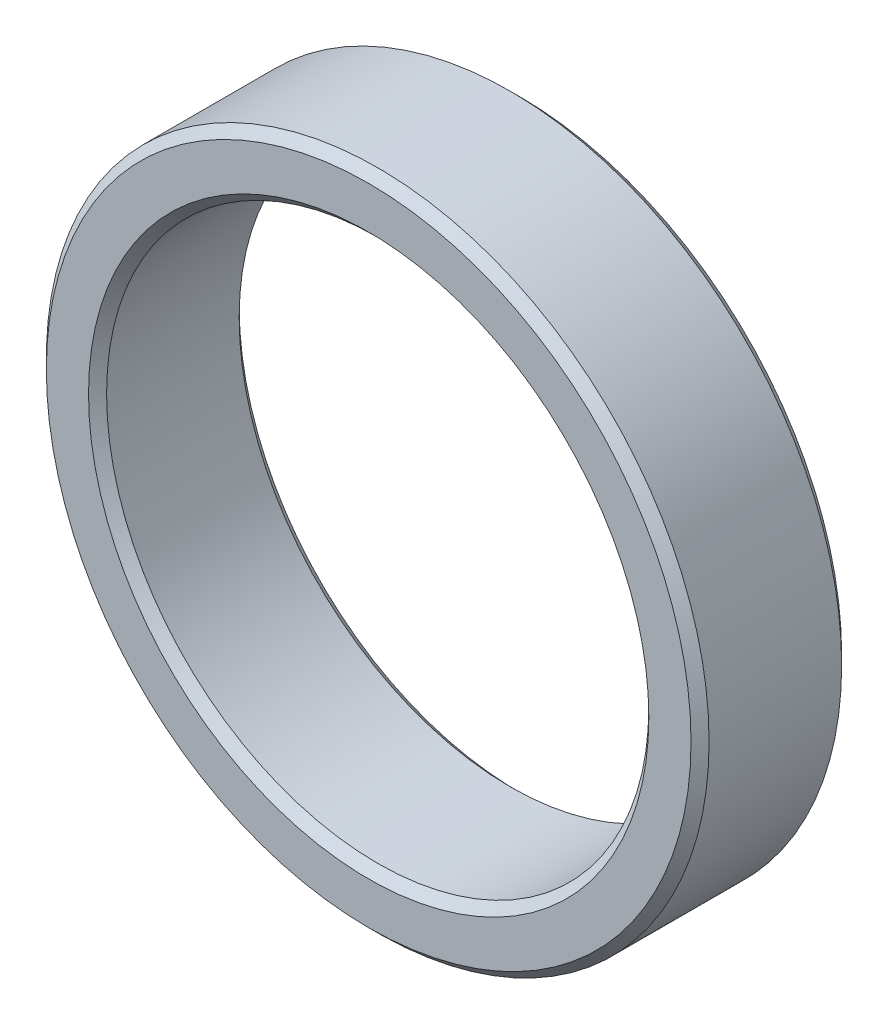
from build123d import *

# Parameters (mm, degrees)
SKETCH_2_R          = 11
EXTRUDE_1_DEPTH     = 5
SKETCH_3_R          = 9
CUT_EXTRUDE_1_DEPTH = 5
CHAMFER_2_SIZE      = 0.3


with BuildPart() as part:
    # 草图2 → 凸台-拉伸1 (new body)
    with BuildSketch(Plane.XY):
        Circle(SKETCH_2_R)
    extrude(amount=EXTRUDE_1_DEPTH)

    # 草图3 → 切除-拉伸1 (cut)
    with BuildSketch(Plane.XY.offset(5)):
        Circle(SKETCH_3_R)
    extrude(amount=-CUT_EXTRUDE_1_DEPTH, mode=Mode.SUBTRACT)

    # 倒角2
    chamfer_2_edges = [part.edges().sort_by_distance(p)[0] for p in [
        (-11, 0, 0),
        (-11, 0, 5),
        (-9, 0, 0),
        (-9, 0, 5),
    ]]
    chamfer(chamfer_2_edges, length=CHAMFER_2_SIZE)


solid = part.part
